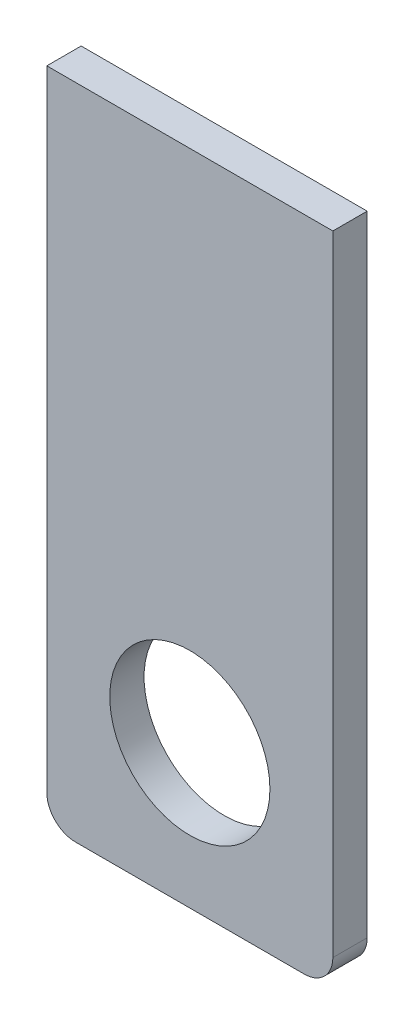
from build123d import *

# Parameters (mm, degrees)
SKETCH1_R           = 14
BOSS_EXTRUDE1_DEPTH = 3


with BuildPart() as part:
    # Sketch1 → Boss-Extrude1 (new, symmetric)
    with BuildSketch(Plane.XY):
        with BuildLine():
            Line((-25, 90), (25, 90))
            Line((25, 90), (25, -20))
            ThreePointArc((25, -20), (23.535533906, -23.535533906), (20, -25))
            Line((20, -25), (-20, -25))
            ThreePointArc((-20, -25), (-23.535533906, -23.535533906), (-25, -20))
            Line((-25, -20), (-25, 90))
        make_face()
        Circle(SKETCH1_R, mode=Mode.SUBTRACT)
    extrude(amount=BOSS_EXTRUDE1_DEPTH, both=True)


solid = part.part
